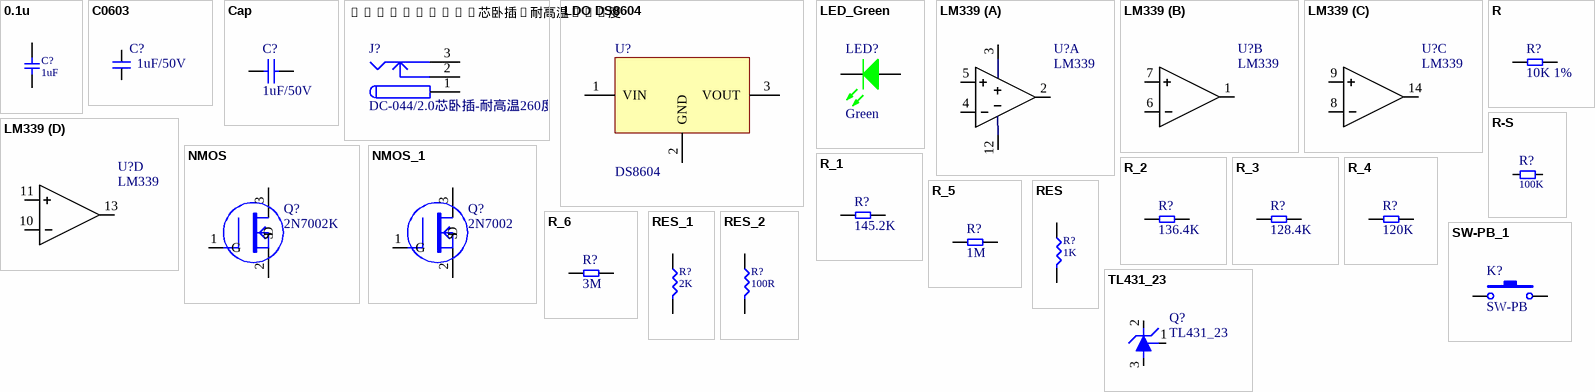
[diagram p0: symbols 0.1u to TL431_23]
# Altium schematic symbol library MISC75799-4.SchLib: 22 symbols
Pins are listed as number, name and electrical type; pins without a type are passive.


## 0.1u
designator C?, comment 1uF
footprint CAP0603 (CAP0402)
footprint 1206C
footprint 0805c
footprint C0603A (SMD capacitor)
pins: 1, 2

## C0603
designator C?, comment 1uF/50V
0603 SMD capacitor
footprint 0805
footprint CAP0603 (CAP0402)
footprint C0603A (SMD capacitor)
pins: 1, 2

## Cap
designator C?, comment 1uF/50V
Capacitor
footprint RAD-0.3 (Radial Cap, Thru-Hole; 2 Leads; 0.3 in Pin Spacing)
simulation model CAP (Capacitor)
signal-integrity model Cap
footprint CAP0603 (CAP0402)
footprint C0402A
footprint C0603A (SMD capacitor)
pins: 1, 2

## DC-044/2.0芯卧插-耐高温260度
designator J?
DC-044 power connector - Yueqing Jinghong
footprint DC-044 (DC power jack through-hole - Yueqing Jinghong)
pins: 1 (power), 2 (power), 3 (power)

## LDO DS8604
designator U?, comment DS8604
LDO
footprint SOT-89
footprint SOT-89-3 (SMD linear regulator)
pins: 1 VIN, 2 GND, 3 VOUT
2 alternate drawings of the same symbol

## LED_Green
designator LED?, comment Green
SMD LED lamp
footprint LED0603A (SMD LED)
footprint LED0805A (SMD LED)
pins: 1 A, 2 K

## LM339
designator U?
footprint SO-14
footprint DIP-14
footprint SOP14L
part A pins: 2 OUT1, 3 VCC, 4 IN1-, 5 IN1+, 12 GND
part B pins: 1 OUT2, 6 IN2-, 7 IN2+
part C pins: 8 IN3-, 9 IN3+, 14 OUT3
part D pins: 10 IN4-, 11 IN4+, 13 OUT4

## NMOS
designator Q?, comment 2N7002K
footprint SOT-23-3
footprint SOT23-3 (SMD IC/MOS*)
pins: 1 G, 2 S, 3 D
2 alternate drawings of the same symbol

## NMOS_1
designator Q?, comment 2N7002
footprint SOT23-3 (SMD IC/MOS*)
footprint SOT-23-3
pins: 1 G, 2 S, 3 D

## R
designator R?, comment 10K 1%
footprint 0805
footprint 1206
footprint R2WD
footprint 2512
footprint 0603
footprint R0603A (SMD resistor)
footprint RES0603 (CAP0402)
pins: 1, 2

## R-S
designator R?, comment 100K
footprint RES0603 (CAP0402)
footprint 0603
footprint R0603A (SMD resistor)
pins: 1, 2

## R_1
designator R?, comment 145.2K
footprint 0805
footprint 1206
footprint R2WD
footprint 2512
footprint 0603
footprint R0603A (SMD resistor)
footprint RES0603 (CAP0402)
pins: 1, 2

## R_2
designator R?, comment 136.4K
footprint 0805
footprint 1206
footprint R2WD
footprint 2512
footprint 0603
footprint R0603A (SMD resistor)
footprint RES0603 (CAP0402)
pins: 1, 2

## R_3
designator R?, comment 128.4K
footprint 0805
footprint 1206
footprint R2WD
footprint 2512
footprint 0603
footprint R0603A (SMD resistor)
footprint RES0603 (CAP0402)
pins: 1, 2

## R_4
designator R?, comment 120K
footprint 0805
footprint 1206
footprint R2WD
footprint 2512
footprint 0603
footprint R0603A (SMD resistor)
footprint RES0603 (CAP0402)
pins: 1, 2

## R_5
designator R?, comment 1M
footprint 0805
footprint 1206
footprint R2WD
footprint 2512
footprint 0603
footprint RES0603 (CAP0402)
footprint R0603A (SMD resistor)
pins: 1, 2

## R_6
designator R?, comment 3M
footprint 0805
footprint 1206
footprint R2WD
footprint 2512
footprint 0603
footprint RES0603 (CAP0402)
footprint R0603A (SMD resistor)
pins: 1, 2

## RES
designator R?, comment 1K
footprint 0603
footprint 0805
footprint 1206
footprint 08053
footprint R0603A (SMD resistor)
footprint RES0603 (CAP0402)
pins: 1, 2

## RES_1
designator R?, comment 2K
footprint RES0805
footprint 0805
footprint 2512
footprint R0805A (SMD resistor)
pins: 1, 2

## RES_2
designator R?, comment 100R
footprint RES0805
footprint 0805
footprint 2512
footprint R0805A (SMD resistor)
pins: 1, 2

## SW-PB_1
designator K?, comment SW-PB
6*6 tactile switch
footprint SW4.5*4.5-SMD
footprint SW4*4
footprint SW6*6*8
footprint SW6X6XH=* (SMD switch)
footprint KEY-TH_4P-L12.0-W12.0-P5.00-LS12.5
footprint SW-SMD_4P-L12.0-W12.0-P5.00-LS15.2
pins: 1, 2

## TL431_23
designator Q?
IC SOT-23
footprint SOT-23-3
footprint SOT23-3 (SMD IC/MOS*)
pins: 1, 2, 3